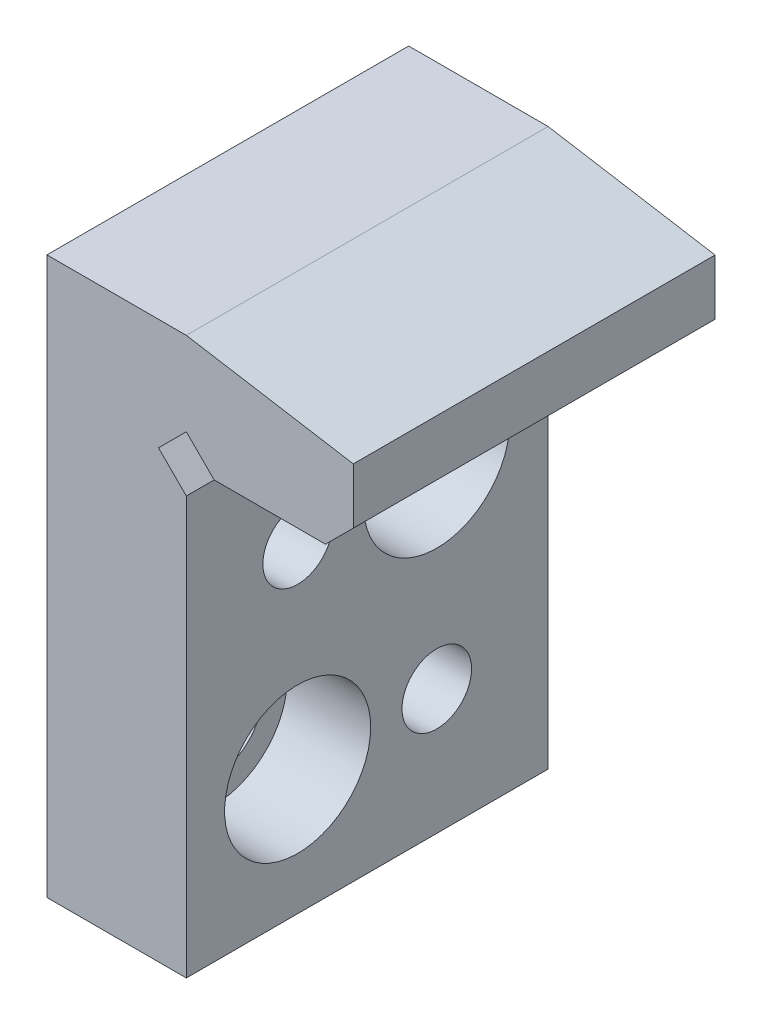
from build123d import *

# Parameters (mm, degrees)
BOSS_EXTRUDE1_DEPTH = 13
SKETCH2_R           = 3.5
SKETCH2_R_2         = 2.5
CUT_EXTRUDE1_DEPTH  = 26
SKETCH3_R           = 5.25
CUT_EXTRUDE2_DEPTH  = 6


with BuildPart() as part:
    # Sketch1 → Boss-Extrude1 (new, symmetric)
    with BuildSketch(Plane.XY):
        Polygon((55.168145317, 40.706551648), (57.168145317, 42.706551648), (57.168145317, 46.706551648), (45.168145317, 48.706551648), (35.15033873, 48.706551648), (35.15033873, 14.706551648), (35.15033873, 8.706551648), (45.168145317, 8.706551648), (45.168145317, 38.706551648), (43.168145317, 40.706551648), (45.168145317, 42.706551648), (47.168145317, 40.706551648), align=None)
    extrude(amount=BOSS_EXTRUDE1_DEPTH, both=True)

    # Sketch2 → Cut-Extrude1 (cut)
    with BuildSketch(Plane(origin=(45.168145317, 0, 0), x_dir=(0, 0, -1), z_dir=(1, 0, 0))):
        with Locations((-5, 17.706551648)):
            Circle(SKETCH2_R)
        with Locations((5, 31.706551648)):
            Circle(SKETCH2_R)
        with Locations((5, 17.706551648)):
            Circle(SKETCH2_R_2)
        with Locations((-5, 31.706551648)):
            Circle(SKETCH2_R_2)
    extrude(amount=-CUT_EXTRUDE1_DEPTH, mode=Mode.SUBTRACT)

    # Sketch3 → Cut-Extrude2 (cut)
    with BuildSketch(Plane(origin=(45.168145317, 0, 0), x_dir=(0, 0, -1), z_dir=(1, 0, 0))):
        with Locations((5, 31.706551648)):
            Circle(SKETCH3_R)
        with Locations((-5, 17.706551648)):
            Circle(SKETCH3_R)
    extrude(amount=-CUT_EXTRUDE2_DEPTH, mode=Mode.SUBTRACT)


solid = part.part
